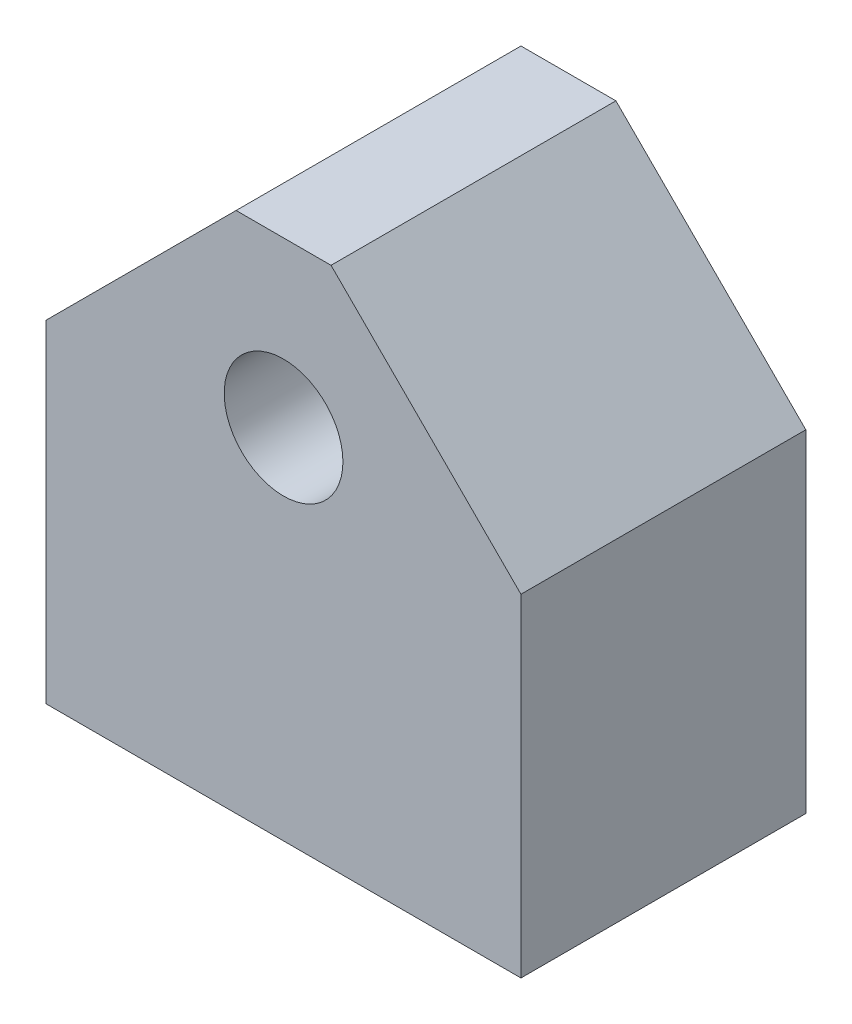
from build123d import *

# Parameters (mm, degrees)
SKETCH_1_W              = 50
SKETCH_1_H              = 55
EXTRUDE_1_DEPTH         = 30
CHAMFER_1_SIZE          = 20
HOLE_WIZARD_M10_1_D     = 8.5
HOLE_WIZARD_M10_1_DEPTH = 24.5
HOLE_WIZARD_M10_1_TIP   = 2.553657631
SKETCH_5_R              = 6.25
CUT_EXTRUDE_1_DEPTH     = 30


with BuildPart() as part:
    # 草图1 → 凸台-拉伸1 (new body)
    with BuildSketch(Plane.XY):
        Rectangle(SKETCH_1_W, SKETCH_1_H)
    extrude(amount=EXTRUDE_1_DEPTH)

    # 倒角1
    chamfer_1_edges = [part.edges().sort_by_distance(p)[0] for p in [
        (-25, 27.5, 15),
        (25, 27.5, 15),
    ]]
    chamfer(chamfer_1_edges, length=CHAMFER_1_SIZE)

    # M10 螺纹孔1
    with Locations(Plane(origin=(0, -27.5, 0), x_dir=(-1, 0, 0), z_dir=(0, -1, 0))):
        with Locations((15, -15), (-15, -15)):
            Hole(HOLE_WIZARD_M10_1_D / 2, depth=HOLE_WIZARD_M10_1_DEPTH)
            with Locations((0, 0, -(HOLE_WIZARD_M10_1_DEPTH + HOLE_WIZARD_M10_1_TIP / 2))):  # 118° drill point
                Cone(0, HOLE_WIZARD_M10_1_D / 2, HOLE_WIZARD_M10_1_TIP, mode=Mode.SUBTRACT)

    # 草图5 → 切除-拉伸1 (cut)
    with BuildSketch(Plane.XY.offset(30)):
        with Locations((0, 10.2)):
            Circle(SKETCH_5_R)
    extrude(amount=-CUT_EXTRUDE_1_DEPTH, mode=Mode.SUBTRACT)


solid = part.part
